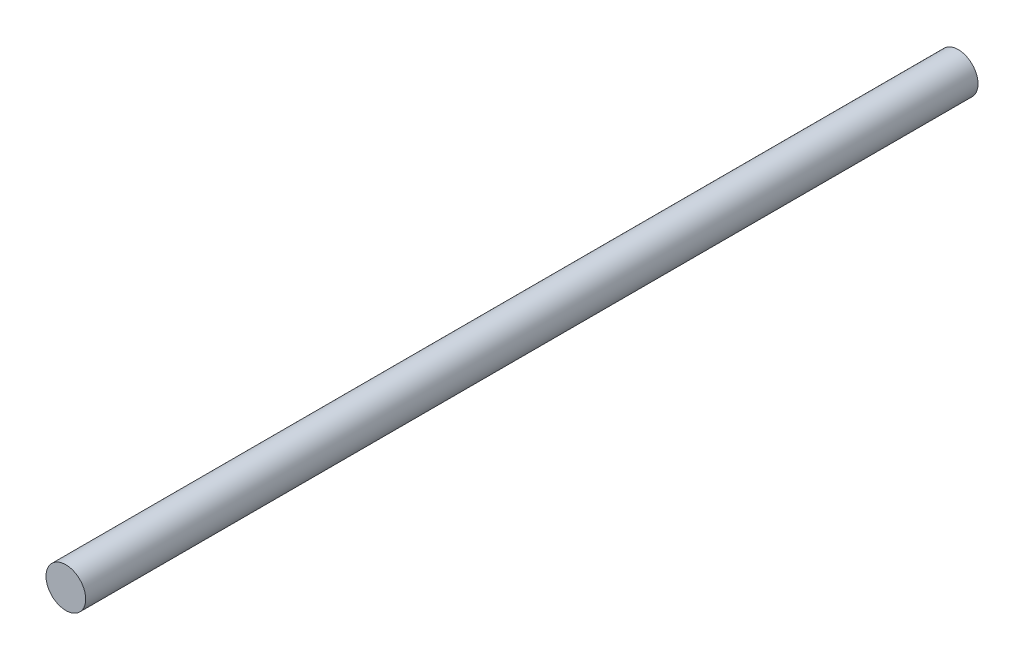
SolidWorks part; units mm, degrees
ref_plane "Front Plane" through (0, 0, 0) normal (0, 0, 1) x (1, 0, 0)
ref_plane "Top Plane" through (0, 0, 0) normal (0, 1, 0) x (1, 0, 0)
ref_plane "Right Plane" through (0, 0, 0) normal (1, 0, 0) x (0, 0, -1)
sketch "Sketch1" plane through (0, 0, 0) normal (0, 0, 1) x (1, 0, 0)
  circle A0 centre (0, 0) radius 2
  dimension "D1" = 4
extrude "Boss-Extrude1" add sketch "Sketch1" along normal blind 90
